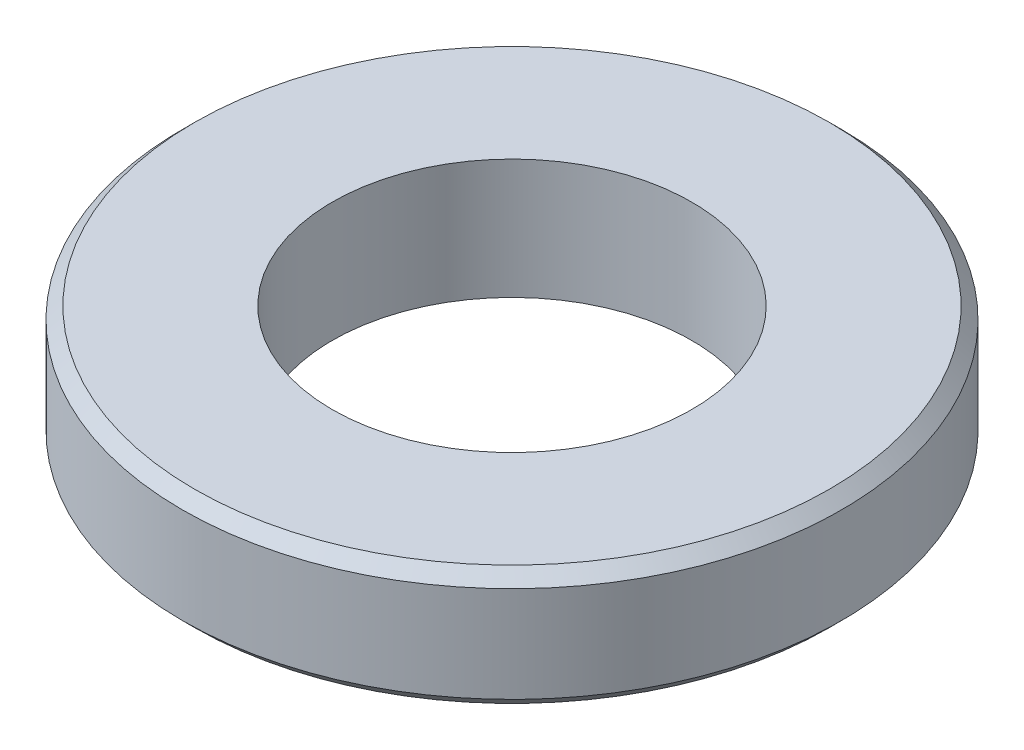
SolidWorks part; units mm, degrees
ref_plane "Front Plane" through (0, 0, 0) normal (0, 0, 1) x (1, 0, 0)
ref_plane "Top Plane" through (0, 0, 0) normal (0, 1, 0) x (1, 0, 0)
ref_plane "Right Plane" through (0, 0, 0) normal (1, 0, 0) x (0, 0, -1)
other "Configuration Table"
sketch "Sketch1" plane through (0, 0, 0) normal (0, 1, 0) x (1, 0, 0)
  circle A0 centre (0, 0) radius 2.75
  circle A1 centre (0, 0) radius 1.5
  dimension "D1" = 3
  dimension "D2" = 5.5
extrude "Boss-Extrude1" add sketch "Sketch1" along normal blind 1
chamfer "Chamfer1" distance 0.1 angle 45 2 edges at (0, 0, 2.75) (0, 1, 2.75)
